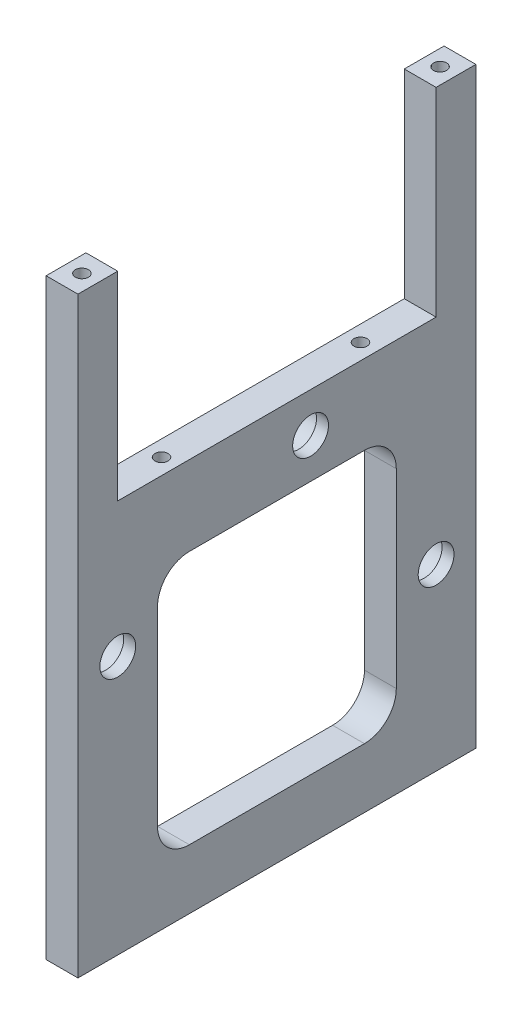
SolidWorks part; units mm, degrees
ref_plane "Front Plane" through (0, 0, 0) normal (0, 0, 1) x (1, 0, 0)
ref_plane "Top Plane" through (0, 0, 0) normal (0, 1, 0) x (1, 0, 0)
ref_plane "Right Plane" through (0, 0, 0) normal (1, 0, 0) x (0, 0, -1)
sketch "Sketch1" plane through (0, 0, 0) normal (1, 0, 0) x (0, 0, -1)
  line L25 (59.943, -63.7659) -> (-40.057, -63.7659)
  line L29 (59.943, -63.7659) -> (59.943, 35.0641)
  line L35 (39.943, -48.7659) -> (-20.057, -48.7659)
  line L36 (-20.057, -48.7659) -> (-20.057, 15.0641)
  line L41 (-40.057, -63.7659) -> (-40.057, 35.0641)
  line L44 (39.943, 15.0641) -> (-20.057, 15.0641)
  line L47 (59.943, 35.0641) -> (-40.057, 35.0641)
  line L49 (39.943, 15.0641) -> (39.943, -48.7659)
  circle A16 centre (-30.057, 1.2341) radius 4.5
  circle A17 centre (18.4005, 25.0641) radius 4.5
  circle A18 centre (49.943, -18.7659) radius 4.5
  dimension "D6" = 54
  dimension "D9" = 80
  dimension "D13" = 10
  dimension "D14" = 45
  dimension "D3" = 54
  dimension "D4" = 65
  dimension "D7" = 9
  dimension "D11" = 10
  dimension "D12" = 10
  dimension "D2" = 10
  dimension "D5" = 10
  dimension "D8" = 10
  dimension "D10" = 15
extrude "Boss-Extrude1" add sketch "Sketch1" along normal blind 8
sketch "Sketch4" plane through (0, 0, 0) normal (-1, 0, 0) x (0, 0, 1)
  circle A0 centre (-18.4005, 25.0641) radius 5.55
  circle A1 centre (30.057, 1.2341) radius 5.55
  circle A2 centre (-49.943, -18.7659) radius 5.55
extrude "Cut-Extrude2" cut sketch "Sketch4" against normal blind 5
sketch "Sketch5" plane through (0, 35.0641, 0) normal (0, 1, 0) x (1, 0, 0)
  line L0 (4, 54.943) -> (4, -35.057) construction
  line L1 (8, 59.943) -> (0, 59.943) construction
  line L2 (0, 59.943) -> (0, -40.057) construction
  line L3 (8, -40.057) -> (0, -40.057) construction
  circle A0 centre (4, 54.943) radius 1
  circle A1 centre (4, -35.057) radius 1
  circle A2 centre (4, 9.943) radius 1
  dimension "D1" = 5
  dimension "D4" = 2
  dimension "D6" = 2
  dimension "D2" = 5
  dimension "D3" = 45
  dimension "D5" = 4
fillet "Fillet2" radius 8 4 edges at (4, 15.0641, 20.057) (4, 15.0641, -39.943) (4, -48.7659, -39.943) (4, -48.7659, 20.057)
sketch "Sketch11" plane through (0, -63.7659, 0) normal (0, -1, 0) x (1, 0, 0)
  line L1 (8, 40.057) -> (0, 40.057) construction
  line L3 (0, -59.943) -> (0, 40.057) construction
  line L4 (4.0019, 30.057) -> (4.0019, -44.943) construction
  circle A0 centre (4.0019, -44.943) radius 1
  circle A1 centre (4.0019, 30.057) radius 1
  circle A2 centre (4.0019, -19.943) radius 1
  circle A3 centre (4.0019, 5.057) radius 1
  dimension "D6" = 10
  dimension "D1" = 25
  dimension "D2" = 4.0019
  dimension "D3" = 25
  dimension "D5" = 25
sketch "Sketch13" plane through (0, 0, 0) normal (-1, 0, 0) x (0, 0, 1)
  line L0 (-18.4005, 25.0641) -> (-10.6505, 25.0641) construction
  line L1 (-18.4005, 25.0641) -> (-26.1505, 25.0641) construction
  line L2 (30.057, 1.2341) -> (30.057, 8.9841) construction
  line L3 (30.057, 1.2341) -> (30.057, -6.5159) construction
  line L4 (-49.943, -18.7659) -> (-49.943, -11.0159) construction
  line L5 (-49.943, -18.7659) -> (-49.943, -26.5159) construction
  dimension "D3" = 7.75
  dimension "D1" = 7.75
  dimension "D2" = 7.75
  dimension "D4" = 7.75
  dimension "D5" = 7.75
  dimension "D6" = 7.75
hole_wizard "M2.5 Tapped Hole1" positions "3DSketch8" profile "Sketch15" tap size "M2.5" standard "GB"
sketch3d "3DSketch8"
  point P0 (0, 25.0641, -26.1505)
  point P3 (0, 25.0641, -10.6505)
  point P6 (0, -11.0159, -49.943)
  point P9 (0, -26.5159, -49.943)
  point P12 (0, 8.9841, 30.057)
  point P15 (0, -6.5159, 30.057)
sketch "Sketch15" plane through (0, 25.0641, -26.1505) normal (0, 1, 0) x (0, 0, 1)
  line L0 (0, 0) -> (0, 6.6159)
  line L1 (0, 6.6159) -> (1.025, 6)
  line L2 (1.025, 6) -> (1.025, 0)
  line L5 (1.025, 0) -> (0, 0)
  line L10 (0, 6.6159) -> (-1.025, 6) construction
  line L11 (0, -6.35) -> (0, 107.95) construction
  dimension "螺纹孔钻头直径" = 2.05
  dimension "螺纹孔钻头深度" = 6
  dimension "导头角度" = 118
cosmetic thread "CosmeticThread24" parameters "D1"=5, "D2"=2.5
cosmetic thread "CosmeticThread25" parameters "D1"=5, "D2"=2.5
cosmetic thread "CosmeticThread26" parameters "D1"=5, "D2"=2.5
cosmetic thread "CosmeticThread27" parameters "D1"=5, "D2"=2.5
cosmetic thread "CosmeticThread28" parameters "D1"=5, "D2"=2.5
cosmetic thread "CosmeticThread29" parameters "D1"=5, "D2"=2.5
extrude "Cut-Extrude3" cut sketch "Sketch11" against normal blind 10
hole_wizard "M4 Tapped Hole1" positions "Sketch16" profile "Sketch18" tap size "M4" standard "GB"
sketch "Sketch16" plane through (0, -63.7659, 0) normal (0, -1, 0) x (-1, 0, 0)
  point P0 (-4.0019, 44.943)
  point P3 (-4.0019, 19.943)
  point P6 (-4.0019, -5.057)
  point P9 (-4.0019, -30.057)
sketch "Sketch18" plane through (4.0019, -63.7659, -44.943) normal (1, 0, 0) x (0, 0, -1)
  line L0 (0, 0) -> (0, 12.4914)
  line L1 (0, 12.4914) -> (1.65, 11.5)
  line L2 (1.65, 11.5) -> (1.65, 0)
  line L5 (1.65, 0) -> (0, 0)
  line L10 (0, 12.4914) -> (-1.65, 11.5) construction
  line L11 (0, -6.35) -> (0, 107.95) construction
  dimension "螺纹孔钻头直径" = 3.3
  dimension "螺纹孔钻头深度" = 11.5
  dimension "导头角度" = 118
cosmetic thread "CosmeticThread30" parameters "D1"=8, "D2"=4
cosmetic thread "CosmeticThread31" parameters "D1"=8, "D2"=4
cosmetic thread "CosmeticThread32" parameters "D1"=8, "D2"=4
cosmetic thread "CosmeticThread33" parameters "D1"=8, "D2"=4
sketch "Sketch21" plane through (0, 35.0641, 0) normal (0, 1, 0) x (1, 0, 0)
  line L0 (8, 59.943) -> (8, -40.057) construction
  line L1 (0, 59.943) -> (8, 59.943)
  line L2 (0, 59.943) -> (0, 49.943)
  line L3 (0, 49.943) -> (8, 49.943)
  line L4 (8, 59.943) -> (8, 49.943)
  line L5 (0, 59.943) -> (0, -40.057) construction
  line L11 (0, -30.057) -> (8, -30.057)
  line L12 (0, -30.057) -> (0, -40.057)
  line L13 (0, -40.057) -> (8, -40.057)
  line L14 (8, -30.057) -> (8, -40.057)
  dimension "D1" = 10
  dimension "D3" = 10
extrude "Boss-Extrude2" add sketch "Sketch21" along normal blind 50
hole_wizard "M4 Tapped Hole5" positions "Sketch29" profile "Sketch30" tap size "M4" standard "GB"
sketch "Sketch29" plane through (0, 85.0641, 0) normal (0, 1, 0) x (1, 0, 0)
  line L0 (8, 59.943) -> (0, 59.943) construction
  line L4 (0, -40.057) -> (8, -40.057) construction
  line L5 (0, -30.057) -> (0, -40.057) construction
  point P0 (4, 54.943)
  point P4 (4, -35.057)
  dimension "D1" = 5
  dimension "D2" = 4
  dimension "D5" = 5
  dimension "D6" = 4
sketch "Sketch30" plane through (4, 85.0641, -54.943) normal (1, 0, 0) x (0, 0, 1)
  line L0 (0, 0) -> (0, 8.9914)
  line L1 (0, 8.9914) -> (1.65, 8)
  line L2 (1.65, 8) -> (1.65, 0)
  line L5 (1.65, 0) -> (0, 0)
  line L10 (0, 8.9914) -> (-1.65, 8) construction
  line L11 (0, -6.35) -> (0, 107.95) construction
  dimension "螺纹孔钻头直径" = 3.3
  dimension "螺纹孔钻头深度" = 8
  dimension "导头角度" = 118
cosmetic thread "CosmeticThread40" parameters "D1"=8, "D2"=4
cosmetic thread "CosmeticThread42" parameters "D1"=8, "D2"=4
hole_wizard "M4 Tapped Hole6" positions "Sketch32" profile "Sketch33" tap size "M4" standard "GB"
sketch "Sketch32" plane through (0, 35.0641, 0) normal (0, 1, 0) x (1, 0, 0)
  line L0 (0, 49.943) -> (0, -30.057) construction
  line L1 (0, 49.943) -> (8, 49.943) construction
  line L2 (8, -30.057) -> (0, -30.057) construction
  point P0 (4, 34.943)
  point P2 (4, -15.057)
  dimension "D1" = 4
  dimension "D2" = 15
  dimension "D3" = 4
  dimension "D4" = 15
sketch "Sketch33" plane through (4, 35.0641, -34.943) normal (1, 0, 0) x (0, 0, 1)
  line L0 (0, 0) -> (0, 8.9914)
  line L1 (0, 8.9914) -> (1.65, 8)
  line L2 (1.65, 8) -> (1.65, 0)
  line L5 (1.65, 0) -> (0, 0)
  line L10 (0, 8.9914) -> (-1.65, 8) construction
  line L11 (0, -6.35) -> (0, 107.95) construction
  dimension "螺纹孔钻头直径" = 3.3
  dimension "螺纹孔钻头深度" = 8
  dimension "导头角度" = 118
cosmetic thread "CosmeticThread43" parameters "D1"=8, "D2"=4
cosmetic thread "CosmeticThread44" parameters "D1"=8, "D2"=4
